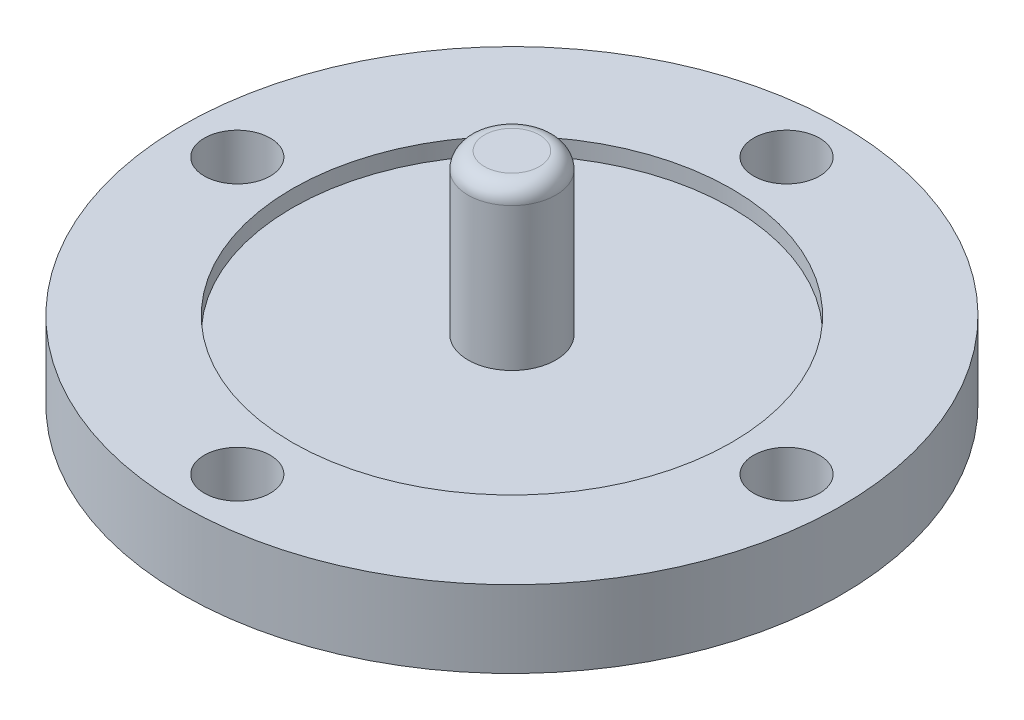
SolidWorks part; units mm, degrees
ref_plane "Front Plane" through (0, 0, 0) normal (0, 0, 1) x (1, 0, 0)
ref_plane "Top Plane" through (0, 0, 0) normal (0, 1, 0) x (1, 0, 0)
ref_plane "Right Plane" through (0, 0, 0) normal (1, 0, 0) x (0, 0, -1)
other "Configuration Table"
sketch "Sketch1" plane through (0, 0, 0) normal (0, 1, 0) x (1, 0, 0)
  circle A0 centre (0, 0) radius 30
  dimension "D1" = 60
extrude "Boss-Extrude1" add sketch "Sketch1" along normal blind 7
sketch "Sketch2" plane through (0, 7, 0) normal (0, 1, 0) x (1, 0, 0)
  circle A0 centre (0, 0) radius 4
  dimension "D1" = 8
extrude "Boss-Extrude2" add sketch "Sketch2" along normal blind 13
sketch "Sketch3" plane through (0, 7, 0) normal (0, 1, 0) x (1, 0, 0)
  circle A0 centre (0, 0) radius 20
  circle A1 centre (0, 0) radius 4
  dimension "D1" = 40
  dimension "D2" = 8
extrude "Cut-Extrude1" cut sketch "Sketch3" against normal blind 1.5
sketch "Sketch4" plane through (0, 0, 0) normal (0, -1, 0) x (-1, 0, 0)
  circle A0 centre (0, 0) radius 25
  point P4 (0, 25)
  point P10 (25, 0)
  point P11 (0, -25)
  point P12 (-25, 0)
  dimension "D1" = 50
  dimension "D2" = 4
hole_wizard "Hole1" positions "Sketch4" profile "Sketch5" legacy end condition through all
sketch "Sketch5" plane through (25, 0, 0) normal (1, 0, 0) x (0, 0, -1)
  line L0 (0, 0) -> (0, 20)
  line L1 (0, 20) -> (3, 20)
  line L2 (3, 20) -> (3, 1.5)
  line L3 (3, 1.5) -> (4.5, 0)
  line L4 (4.5, 0) -> (0, 0)
  line L5 (0, -6.4453) -> (0, 115.525) construction
  line L6 (-3, 1.5) -> (-4.5, 0) construction
  dimension "直径" = 6
  dimension "深度" = 20
  dimension "锥坑角度" = 90
  dimension "锥坑直径" = 9
fillet "Fillet1" radius 1.5 1 edges at (0, 20, 4)
